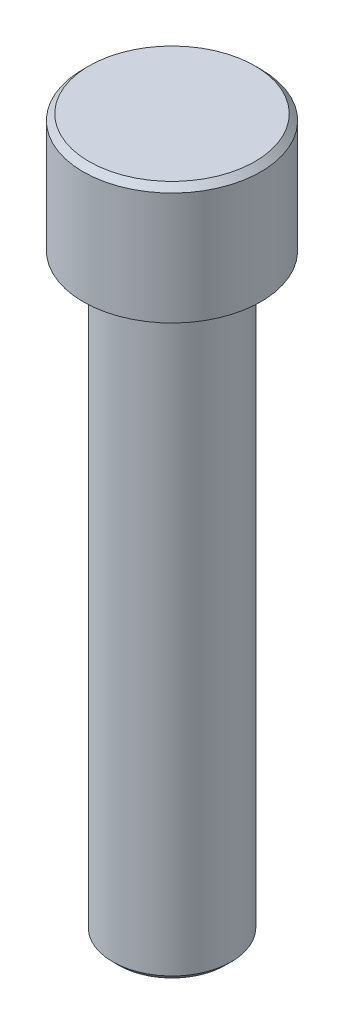
from build123d import *

# Parameters (mm, degrees)
SKETCH_1_R      = 5
EXTRUDE_1_DEPTH = 25
SKETCH_2_R      = 7.5
EXTRUDE_2_DEPTH = 10
CHAMFER_1_SIZE  = 0.5


with BuildPart() as part:
    # 草图1 → 凸台-拉伸1 (new, symmetric)
    with BuildSketch(Plane(origin=(0, 0, 0), x_dir=(1, 0, 0), z_dir=(0, 1, 0))):
        with Locations(Location((0, 0, 0), (0, 0, 270))):
            Circle(SKETCH_1_R)
    extrude(amount=EXTRUDE_1_DEPTH, both=True)

    # 草图2 → 凸台-拉伸2 (add)
    with BuildSketch(Plane(origin=(0, 25, 0), x_dir=(1, 0, 0), z_dir=(0, 1, 0))):
        with Locations(Location((0, 0, 0), (0, 0, 270))):
            Circle(SKETCH_2_R)
    extrude(amount=EXTRUDE_2_DEPTH)

    # 倒角1
    chamfer_1_edges = [part.edges().sort_by_distance(p)[0] for p in [
        (0, -25, -5),
        (0, 35, -7.5),
    ]]
    chamfer(chamfer_1_edges, length=CHAMFER_1_SIZE)


solid = part.part
